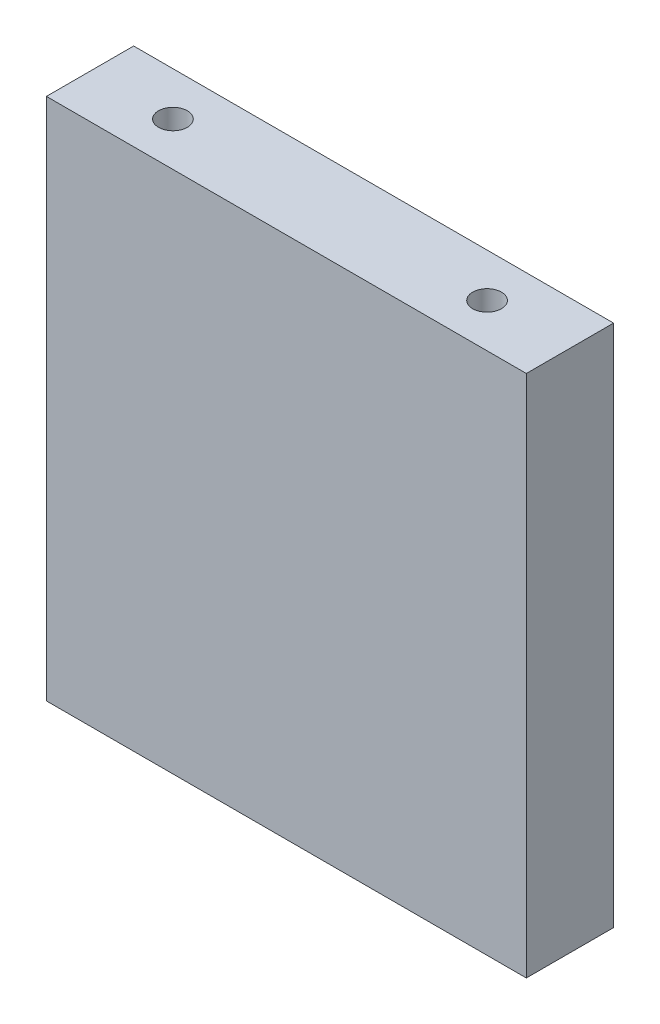
SolidWorks part; units mm, degrees
material "6061铝"
ref_plane "前视基准面" through (0, 0, 0) normal (0, 0, 1) x (1, 0, 0)
ref_plane "上视基准面" through (0, 0, 0) normal (0, 1, 0) x (1, 0, 0)
ref_plane "右视基准面" through (0, 0, 0) normal (1, 0, 0) x (0, 0, -1)
sketch "草图1" plane through (0, 0, 0) normal (0, 0, 1) x (1, 0, 0)
  line L1 (-27.5, 30) -> (27.5, 30)
  line L2 (-27.5, 30) -> (-27.5, -30)
  line L3 (-27.5, -30) -> (27.5, -30)
  line L4 (27.5, 30) -> (27.5, -30)
  line L5 (-27.5, 30) -> (27.5, -30) construction
  line L6 (-27.5, -30) -> (27.5, 30) construction
  point P0 (0, 0)
  dimension "D1" = 55
  dimension "D2" = 60
extrude "凸台-拉伸1" add sketch "草图1" along normal mid plane 10
hole_wizard "M4 螺纹孔1" positions "草图2" profile "草图4" tap size "M4" standard "GB"
sketch "草图2" plane through (0, -30, 0) normal (0, -1, 0) x (-1, 0, 0)
  line L0 (0, 0) -> (0, 8.7748) construction
  point P0 (-18, 0)
  point P7 (18, 0)
  dimension "D1" = 36
cosmetic thread "孔螺蚊线1" parameters "D1"=8, "D2"=4
cosmetic thread "孔螺蚊线2" parameters "D1"=8, "D2"=4
sketch "草图4" plane through (18, -30, 0) normal (1, 0, 0) x (0, 0, -1)
  line L0 (0, 0) -> (0, 12.4914)
  line L1 (0, 12.4914) -> (1.65, 11.5)
  line L2 (1.65, 11.5) -> (1.65, 0)
  line L5 (1.65, 0) -> (0, 0)
  line L10 (0, 12.4914) -> (-1.65, 11.5) construction
  line L11 (0, -6.35) -> (0, 107.95) construction
  dimension "螺纹孔钻头直径" = 3.3
  dimension "螺纹孔钻头深度" = 11.5
  dimension "导头角度" = 118
mirror "镜向1" about plane through (0, 0, 0) normal (0, 1, 0) of "M4 螺纹孔1"
